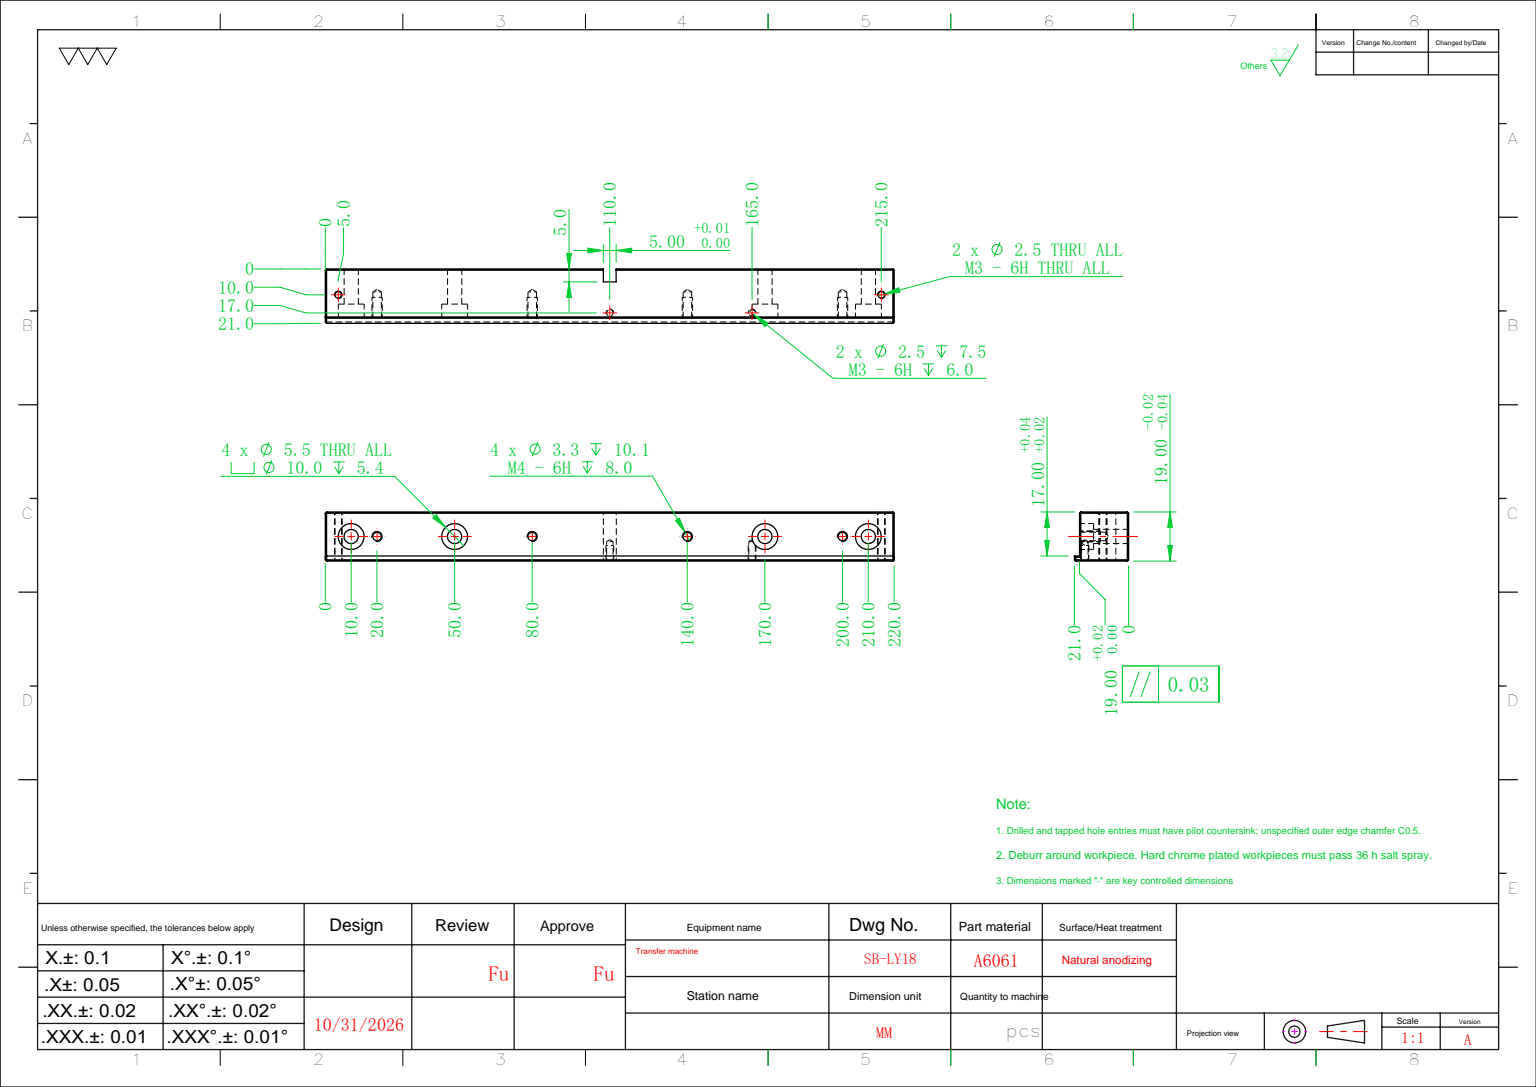
from build123d import *

# Parameters (mm, degrees)
SKETCH_1_W                   = 220
SKETCH_1_H                   = 21
EXTRUDE_1_DEPTH              = 19
SKETCH_2_W                   = 220
SKETCH_2_H                   = 15
CUT_EXTRUDE_1_DEPTH          = 2
HOLE_WIZARD_M4_1_D           = 3.3
HOLE_WIZARD_M4_1_DEPTH       = 10.1
HOLE_WIZARD_M4_1_TIP         = 0.991420021
HOLE_WIZARD_M5_1_D           = 5.5
HOLE_WIZARD_M5_1_CBORE_D     = 10
HOLE_WIZARD_M5_1_CBORE_DEPTH = 5.4
SKETCH_7_W                   = 5
SKETCH_7_H                   = 5
CUT_EXTRUDE_2_DEPTH          = 113.12158579
HOLE_WIZARD_M3_1_D           = 2.5
HOLE_WIZARD_M3_1_DEPTH       = 7.5
HOLE_WIZARD_M3_1_TIP         = 0.751075774
SKETCH_12_W                  = 2
SKETCH_12_H                  = 2
CUT_EXTRUDE_3_DEPTH          = 222.06842832
CHAMFER_1_SIZE               = 0.5
HOLE_WIZARD_M3_2_D           = 2.5


with BuildPart() as part:
    # 草图1 → 凸台-拉伸1 (new body)
    with BuildSketch(Plane.XY):
        Rectangle(SKETCH_1_W, SKETCH_1_H)
    extrude(amount=EXTRUDE_1_DEPTH)

    # 草图2 → 切除-拉伸1 (cut)
    with BuildSketch(Plane.XZ.offset(10.5)):
        with Locations((0, 9.5)):
            Rectangle(SKETCH_2_W, SKETCH_2_H)
    extrude(amount=-CUT_EXTRUDE_1_DEPTH, mode=Mode.SUBTRACT)

    # M4 螺纹孔1
    with Locations(Plane(origin=(0, -8.5, 0), x_dir=(-1, 0, 0), z_dir=(0, -1, 0))):
        with Locations((-90, -9.5), (-30, -9.5), (30, -9.5), (90, -9.5)):
            Hole(HOLE_WIZARD_M4_1_D / 2, depth=HOLE_WIZARD_M4_1_DEPTH)
            with Locations((0, 0, -(HOLE_WIZARD_M4_1_DEPTH + HOLE_WIZARD_M4_1_TIP / 2))):  # 118° drill point
                Cone(0, HOLE_WIZARD_M4_1_D / 2, HOLE_WIZARD_M4_1_TIP, mode=Mode.SUBTRACT)

    # M5 六角凹头螺钉的柱形沉头孔1 (through all)
    with Locations(Plane(origin=(0, -8.5, 0), x_dir=(-1, 0, 0), z_dir=(0, -1, 0))):
        with Locations((-100, -9.5), (100, -9.5), (60, -9.5), (-60, -9.5)):
            CounterBoreHole(HOLE_WIZARD_M5_1_D / 2, HOLE_WIZARD_M5_1_CBORE_D / 2, HOLE_WIZARD_M5_1_CBORE_DEPTH)

    # 草图7 → 切除-拉伸2 (cut, through all)
    with BuildSketch(Plane.XY.offset(19)):
        with Locations((0, 8)):
            Rectangle(SKETCH_7_W, SKETCH_7_H)
    extrude(amount=-CUT_EXTRUDE_2_DEPTH, mode=Mode.SUBTRACT)

    # M3 螺纹孔1
    with Locations(Plane(origin=(0, 0, 0), x_dir=(-1, 0, 0), z_dir=(0, 0, -1))):
        with Locations((-55, -6.5), (0, -6.5)):
            Hole(HOLE_WIZARD_M3_1_D / 2, depth=HOLE_WIZARD_M3_1_DEPTH)
            with Locations((0, 0, -(HOLE_WIZARD_M3_1_DEPTH + HOLE_WIZARD_M3_1_TIP / 2))):  # 118° drill point
                Cone(0, HOLE_WIZARD_M3_1_D / 2, HOLE_WIZARD_M3_1_TIP, mode=Mode.SUBTRACT)

    # 草图12 → 切除-拉伸3 (cut, through all)
    with BuildSketch(Plane(origin=(110, 0, 0), x_dir=(0, 0, -1), z_dir=(1, 0, 0))):
        with Locations((-18, -9.5)):
            Rectangle(SKETCH_12_W, SKETCH_12_H)
    extrude(amount=-CUT_EXTRUDE_3_DEPTH, mode=Mode.SUBTRACT)

    # 倒角1
    chamfer_1_edges = [part.edges().sort_by_distance(p)[0] for p in [
        (-110, 1, 19),
        (110, 1, 19),
        (0, -8.5, 19),
        (110, -10.5, 1),
        (-110, -10.5, 1),
        (110, -8.5, 10.5),
        (110, -9.5, 2),
        (-110, -8.5, 10.5),
        (-110, -9.5, 2),
        (0, -10.5, 0),
        (-110, 0, 0),
        (56.25, 10.5, 0),
        (110, 0, 0),
        (56.25, 10.5, 19),
        (-110, 10.5, 9.5),
        (110, 10.5, 9.5),
        (-56.25, 10.5, 0),
        (-56.25, 10.5, 19),
    ]]
    chamfer(chamfer_1_edges, length=CHAMFER_1_SIZE)

    # M3 螺纹孔2 (through all)
    with Locations(Plane(origin=(0, 0, 0), x_dir=(-1, 0, 0), z_dir=(0, 0, -1))):
        with Locations((105, 0.5), (-105, 0.5)):
            Hole(HOLE_WIZARD_M3_2_D / 2)


solid = part.part
